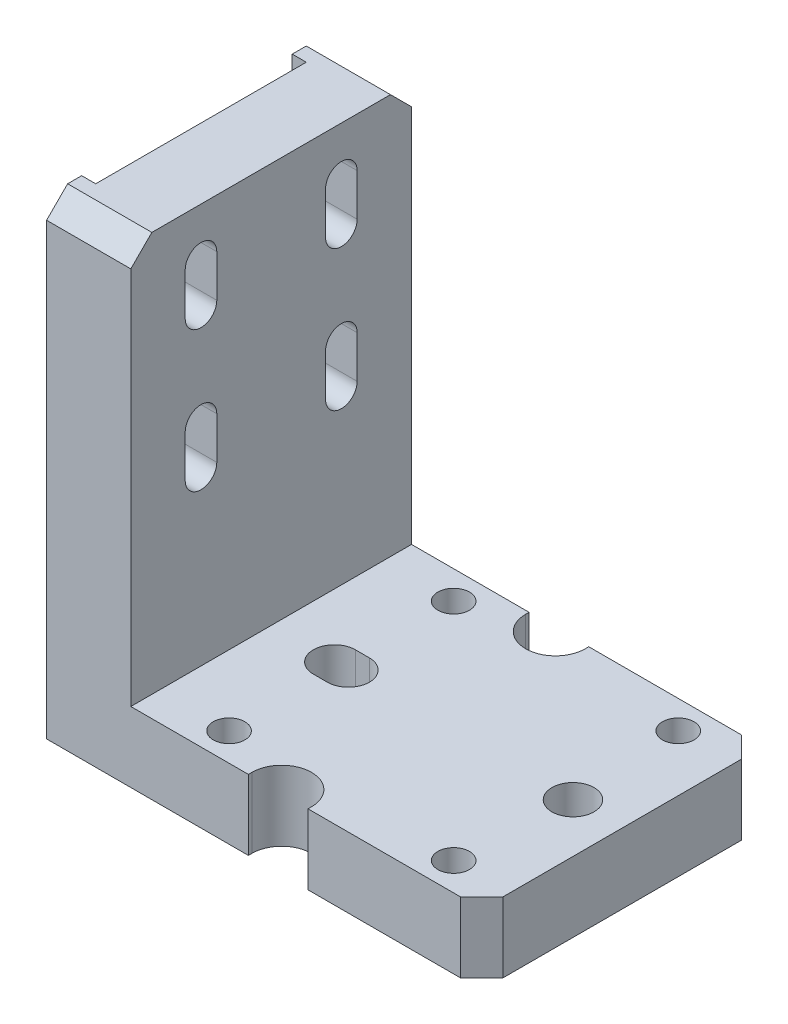
SolidWorks part; units mm, degrees
ref_plane "Front Plane" through (0, 0, 0) normal (0, 0, 1) x (1, 0, 0)
ref_plane "Top Plane" through (0, 0, 0) normal (0, 1, 0) x (1, 0, 0)
ref_plane "Right Plane" through (0, 0, 0) normal (1, 0, 0) x (0, 0, -1)
sketch "Sketch1" plane through (0, 0, 0) normal (0, 0, 1) x (1, 0, 0)
  line L1 (-31, 33.5) -> (31, 33.5)
  line L2 (-31, 33.5) -> (-31, -33.5)
  line L3 (-31, -33.5) -> (31, -33.5)
  line L4 (31, 33.5) -> (31, -33.5)
  line L5 (-31, 33.5) -> (31, -33.5) construction
  line L6 (-31, -33.5) -> (31, 33.5) construction
  point P0 (0, 0)
  dimension "D1" = 62
  dimension "D2" = 67
extrude "Boss-Extrude1" add sketch "Sketch1" along normal mid plane 40
sketch "Sketch2" plane through (0, 0, 20) normal (0, 0, 1) x (1, 0, 0)
  line L0 (-31, 33.5) -> (-31, -33.5) construction
  line L1 (31, 33.5) -> (-19, 33.5)
  line L2 (31, 33.5) -> (31, -23.5)
  line L3 (31, -23.5) -> (-19, -23.5)
  line L4 (-19, 33.5) -> (-19, -23.5)
  line L5 (-31, -33.5) -> (31, -33.5) construction
  dimension "D1" = 12
  dimension "D2" = 10
extrude "Cut-Extrude1" cut sketch "Sketch2" against normal through all
sketch "Sketch3" plane through (0, 33.5, 0) normal (0, 1, 0) x (1, 0, 0)
  line L0 (-31, -20) -> (-31, 20) construction
  line L1 (-31, 15) -> (-29, 15)
  line L2 (-31, 15) -> (-31, -15)
  line L3 (-31, -15) -> (-29, -15)
  line L4 (-29, 15) -> (-29, -15)
  line L5 (0, 0) -> (-37.0643, 0) construction
  dimension "D1" = 30
  dimension "D2" = 2
extrude "Cut-Extrude2" cut sketch "Sketch3" against normal through all
sketch "Sketch4" plane through (-19, 0, 0) normal (1, 0, 0) x (0, 0, -1)
  line L0 (-10, 26.5) -> (-10, 20.5) construction
  line L1 (-7.75, 26.5) -> (-7.75, 20.5)
  line L2 (-12.25, 26.5) -> (-12.25, 20.5)
  line L3 (-10, 6.5) -> (-10, 0.5) construction
  line L4 (-7.75, 6.5) -> (-7.75, 0.5)
  line L5 (-12.25, 6.5) -> (-12.25, 0.5)
  line L6 (10, 26.5) -> (10, 20.5) construction
  line L7 (12.25, 26.5) -> (12.25, 20.5)
  line L8 (7.75, 26.5) -> (7.75, 20.5)
  line L9 (10, 6.5) -> (10, 0.5) construction
  line L10 (12.25, 6.5) -> (12.25, 0.5)
  line L11 (7.75, 6.5) -> (7.75, 0.5)
  line L12 (0, 0) -> (0, 47.3156) construction
  line L13 (20, 33.5) -> (-20, 33.5) construction
  arc A0 (-7.75, 26.5) -> (-12.25, 26.5) centre (-10, 26.5) ccw
  arc A1 (-12.25, 20.5) -> (-7.75, 20.5) centre (-10, 20.5) ccw
  arc A2 (-7.75, 6.5) -> (-12.25, 6.5) centre (-10, 6.5) ccw
  arc A3 (-12.25, 0.5) -> (-7.75, 0.5) centre (-10, 0.5) ccw
  arc A4 (12.25, 26.5) -> (7.75, 26.5) centre (10, 26.5) ccw
  arc A5 (7.75, 20.5) -> (12.25, 20.5) centre (10, 20.5) ccw
  arc A6 (12.25, 6.5) -> (7.75, 6.5) centre (10, 6.5) ccw
  arc A7 (7.75, 0.5) -> (12.25, 0.5) centre (10, 0.5) ccw
  point P2 (-10, 23.5)
  point P7 (-10, 3.5)
  point P14 (10, 23.5)
  point P21 (10, 3.5)
  dimension "D1" = 4.5
  dimension "D2" = 6
  dimension "D3" = 20
  dimension "D4" = 20
  dimension "D5" = 10
extrude "Cut-Extrude3" cut sketch "Sketch4" against normal through all
hole_wizard "Ø4.5 (4.5) Diameter Hole1" positions "Sketch6" profile "Sketch5" hole size "Ø4.5" standard "Gb" end condition through all
sketch "Sketch6" plane through (0, -23.5, 0) normal (0, 1, 0) x (1, 0, 0)
  line L0 (0, 0) -> (35.2511, 0) construction
  line L2 (-19, 20) -> (-19, -20) construction
  point P0 (-9, 16)
  point P2 (-9, -16)
  point P4 (23, -16)
  point P6 (23, 16)
  dimension "D1" = 32
  dimension "D2" = 32
  dimension "D3" = 10
sketch "Sketch5" plane through (-9, -23.5, -16) normal (1, 0, 0) x (0, 0, 1)
  line L0 (0, 0) -> (0, 10)
  line L1 (0, 10) -> (2.25, 10)
  line L2 (2.25, 10) -> (2.25, 0)
  line L5 (2.25, 0) -> (0, 0)
  line L11 (0, -6.35) -> (0, 107.95) construction
  dimension "通孔孔直径" = 4.5
  dimension "通孔孔深度" = 10
sketch "Sketch7" plane through (0, -23.5, 0) normal (0, 1, 0) x (1, 0, 0)
  line L0 (-10, 0) -> (-8, 0) construction
  line L1 (-10, 3) -> (-8, 3)
  line L2 (-10, -3) -> (-8, -3)
  line L3 (-19, 20) -> (-19, -20) construction
  arc A0 (-10, 3) -> (-10, -3) centre (-10, 0) ccw
  arc A1 (-8, -3) -> (-8, 3) centre (-8, 0) ccw
  circle A2 centre (24, 0) radius 3
  point P2 (-9, 0)
  dimension "D2" = 6
  dimension "D1" = 6
  dimension "D3" = 33
  dimension "D4" = 10
  dimension "D5" = 2
extrude "Cut-Extrude4" cut sketch "Sketch7" against normal through all
chamfer "Chamfer1" distance 3 angle 45 4 edges at (31, -28.5, -20) (31, -28.5, 20) (-25, 33.5, -20) (-25, 33.5, 20)
sketch "Sketch8" plane through (0, -23.5, 0) normal (0, 1, 0) x (1, 0, 0)
  line L0 (2, -19.5) -> (2, -27.0275) construction
  line L1 (6.25, -19.5) -> (6.25, -27.0275)
  line L2 (-2.25, -19.5) -> (-2.25, -27.0275)
  line L3 (2, 19.5) -> (2, 27.0275) construction
  line L4 (-2.25, 19.5) -> (-2.25, 27.0275)
  line L5 (6.25, 19.5) -> (6.25, 27.0275)
  line L6 (31, 17) -> (31, -17) construction
  line L7 (0, 0) -> (38.6154, 0) construction
  arc A0 (6.25, -19.5) -> (-2.25, -19.5) centre (2, -19.5) ccw
  arc A1 (-2.25, -27.0275) -> (6.25, -27.0275) centre (2, -27.0275) ccw
  arc A2 (-2.25, 19.5) -> (6.25, 19.5) centre (2, 19.5) ccw
  arc A3 (6.25, 27.0275) -> (-2.25, 27.0275) centre (2, 27.0275) ccw
  point P2 (2, -23.2637)
  point P7 (2, 23.2637)
  dimension "D1" = 8.5
  dimension "D2" = 29
  dimension "D3" = 39
extrude "Cut-Extrude5" cut sketch "Sketch8" against normal through all
